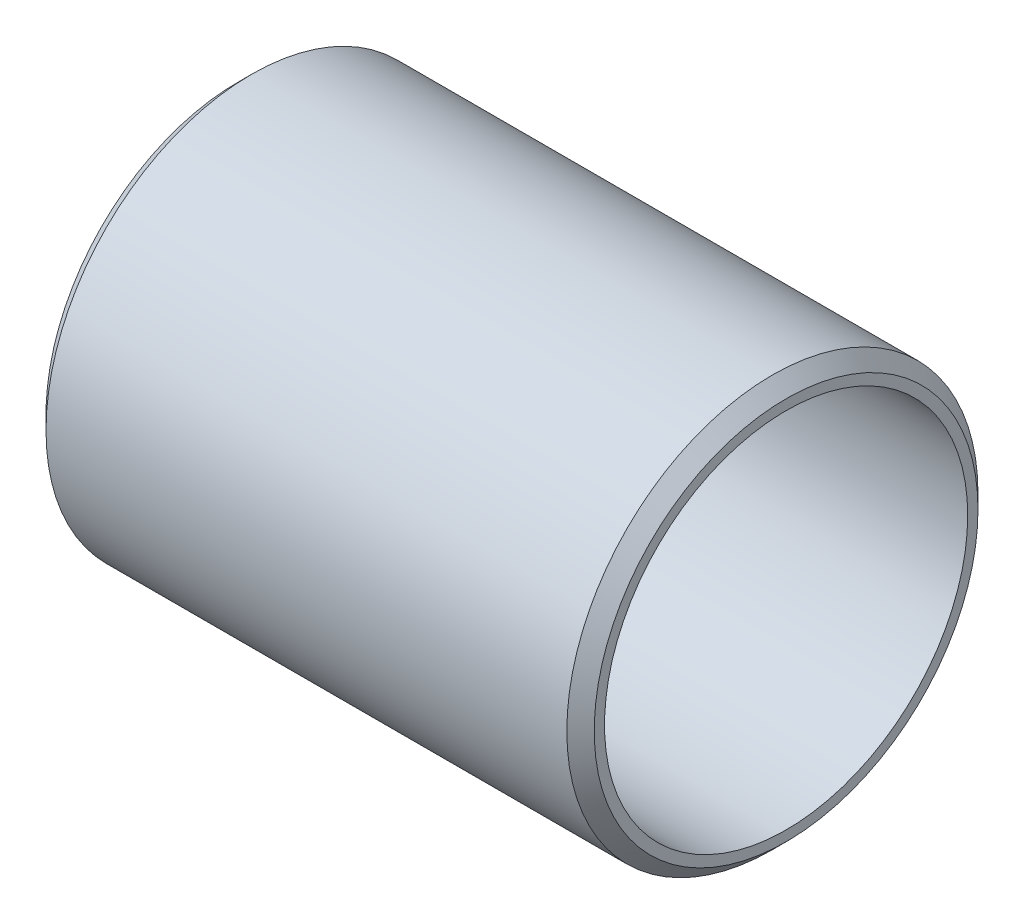
from build123d import *

# Parameters (mm, degrees)
SKETCH_1_R      = 30
SKETCH_1_R_2    = 26.5
EXTRUDE_1_DEPTH = 80
CHAMFER_1_SIZE  = 2


with BuildPart() as part:
    # 草图1 → 拉伸-薄壁1 (new body)
    with BuildSketch(Plane(origin=(0, 0, 0), x_dir=(0, 0, -1), z_dir=(1, 0, 0))):
        Circle(SKETCH_1_R)
        Circle(SKETCH_1_R_2, mode=Mode.SUBTRACT)
    extrude(amount=EXTRUDE_1_DEPTH)

    # 倒角1
    chamfer_1_edges = [part.edges().sort_by_distance(p)[0] for p in [
        (0, 0, 30),
        (80, 0, 30),
    ]]
    chamfer(chamfer_1_edges, length=CHAMFER_1_SIZE)


solid = part.part
